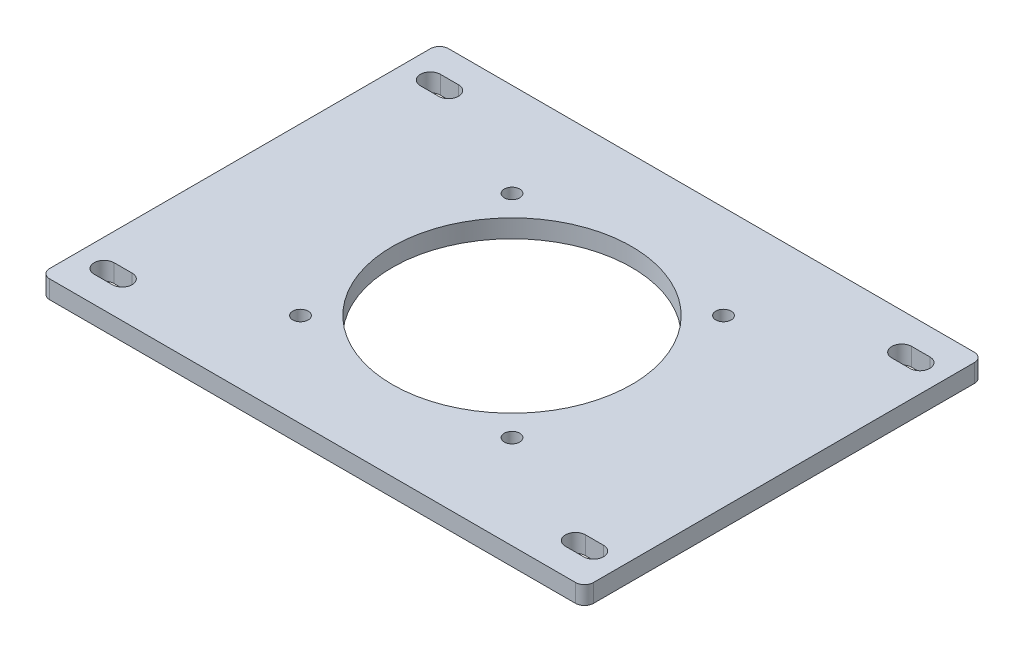
from build123d import *

# Parameters (mm, degrees)
SKETCH1_W              = 300
SKETCH1_H              = 220
BOSS_EXTRUDE1_DEPTH    = 10
SKETCH3_R              = 66
CUT_EXTRUDE1_DEPTH     = 187.279360102
M10_TAPPED_HOLE1_D     = 8.5
M10_TAPPED_HOLE1_DEPTH = 24.5
M10_TAPPED_HOLE1_TIP   = 2.553657631
CUT_EXTRUDE2_DEPTH     = 187.279360102
FILLET1_R              = 5


with BuildPart() as part:
    # Sketch1 → Boss-Extrude1 (new body)
    with BuildSketch(Plane(origin=(0, 0, 0), x_dir=(1, 0, 0), z_dir=(0, 1, 0))):
        Rectangle(SKETCH1_W, SKETCH1_H)
    extrude(amount=BOSS_EXTRUDE1_DEPTH)

    # Sketch3 → Cut-Extrude1 (cut, through all)
    with BuildSketch(Plane(origin=(0, 10, 0), x_dir=(1, 0, 0), z_dir=(0, 1, 0))):
        with Locations(Location((0, 0, 0), (0, 0, 270))):
            Circle(SKETCH3_R)
    extrude(amount=-CUT_EXTRUDE1_DEPTH, mode=Mode.SUBTRACT)

    # M10 Tapped Hole1
    with Locations(Plane(origin=(0, 10, 0), x_dir=(1, 0, 0), z_dir=(0, 1, 0))):
        with Locations((-58.336309448, -58.336309448), (-58.336309448, 58.336309448), (58.336309448, 58.336309448), (58.336309448, -58.336309448)):
            Hole(M10_TAPPED_HOLE1_D / 2, depth=M10_TAPPED_HOLE1_DEPTH)
            with Locations((0, 0, -(M10_TAPPED_HOLE1_DEPTH + M10_TAPPED_HOLE1_TIP / 2))):  # 118° drill point
                Cone(0, M10_TAPPED_HOLE1_D / 2, M10_TAPPED_HOLE1_TIP, mode=Mode.SUBTRACT)

    # Sketch6 → Cut-Extrude2 (cut, through all)
    with BuildSketch(Plane(origin=(0, 10, 0), x_dir=(1, 0, 0), z_dir=(0, 1, 0))):
        with BuildLine():
            Line((-135, 95.5), (-125, 95.5))
            ThreePointArc((-125, 95.5), (-119.5, 90), (-125, 84.5))
            Line((-125, 84.5), (-135, 84.5))
            ThreePointArc((-135, 84.5), (-140.5, 90), (-135, 95.5))
        make_face()
        with BuildLine():
            Line((135, 95.5), (125, 95.5))
            ThreePointArc((125, 95.5), (119.5, 90), (125, 84.5))
            Line((125, 84.5), (135, 84.5))
            ThreePointArc((135, 84.5), (140.5, 90), (135, 95.5))
        make_face()
        with BuildLine():
            Line((135, -95.5), (125, -95.5))
            ThreePointArc((125, -95.5), (119.5, -90), (125, -84.5))
            Line((125, -84.5), (135, -84.5))
            ThreePointArc((135, -84.5), (140.5, -90), (135, -95.5))
        make_face()
        with BuildLine():
            Line((-135, -95.5), (-125, -95.5))
            ThreePointArc((-125, -95.5), (-119.5, -90), (-125, -84.5))
            Line((-125, -84.5), (-135, -84.5))
            ThreePointArc((-135, -84.5), (-140.5, -90), (-135, -95.5))
        make_face()
    extrude(amount=-CUT_EXTRUDE2_DEPTH, mode=Mode.SUBTRACT)

    # Fillet1
    fillet1_edges = [part.edges().sort_by_distance(p)[0] for p in [
        (150, 5, 110),
        (-150, 5, 110),
        (-150, 5, -110),
        (150, 5, -110),
    ]]
    fillet(fillet1_edges, radius=FILLET1_R)


solid = part.part
